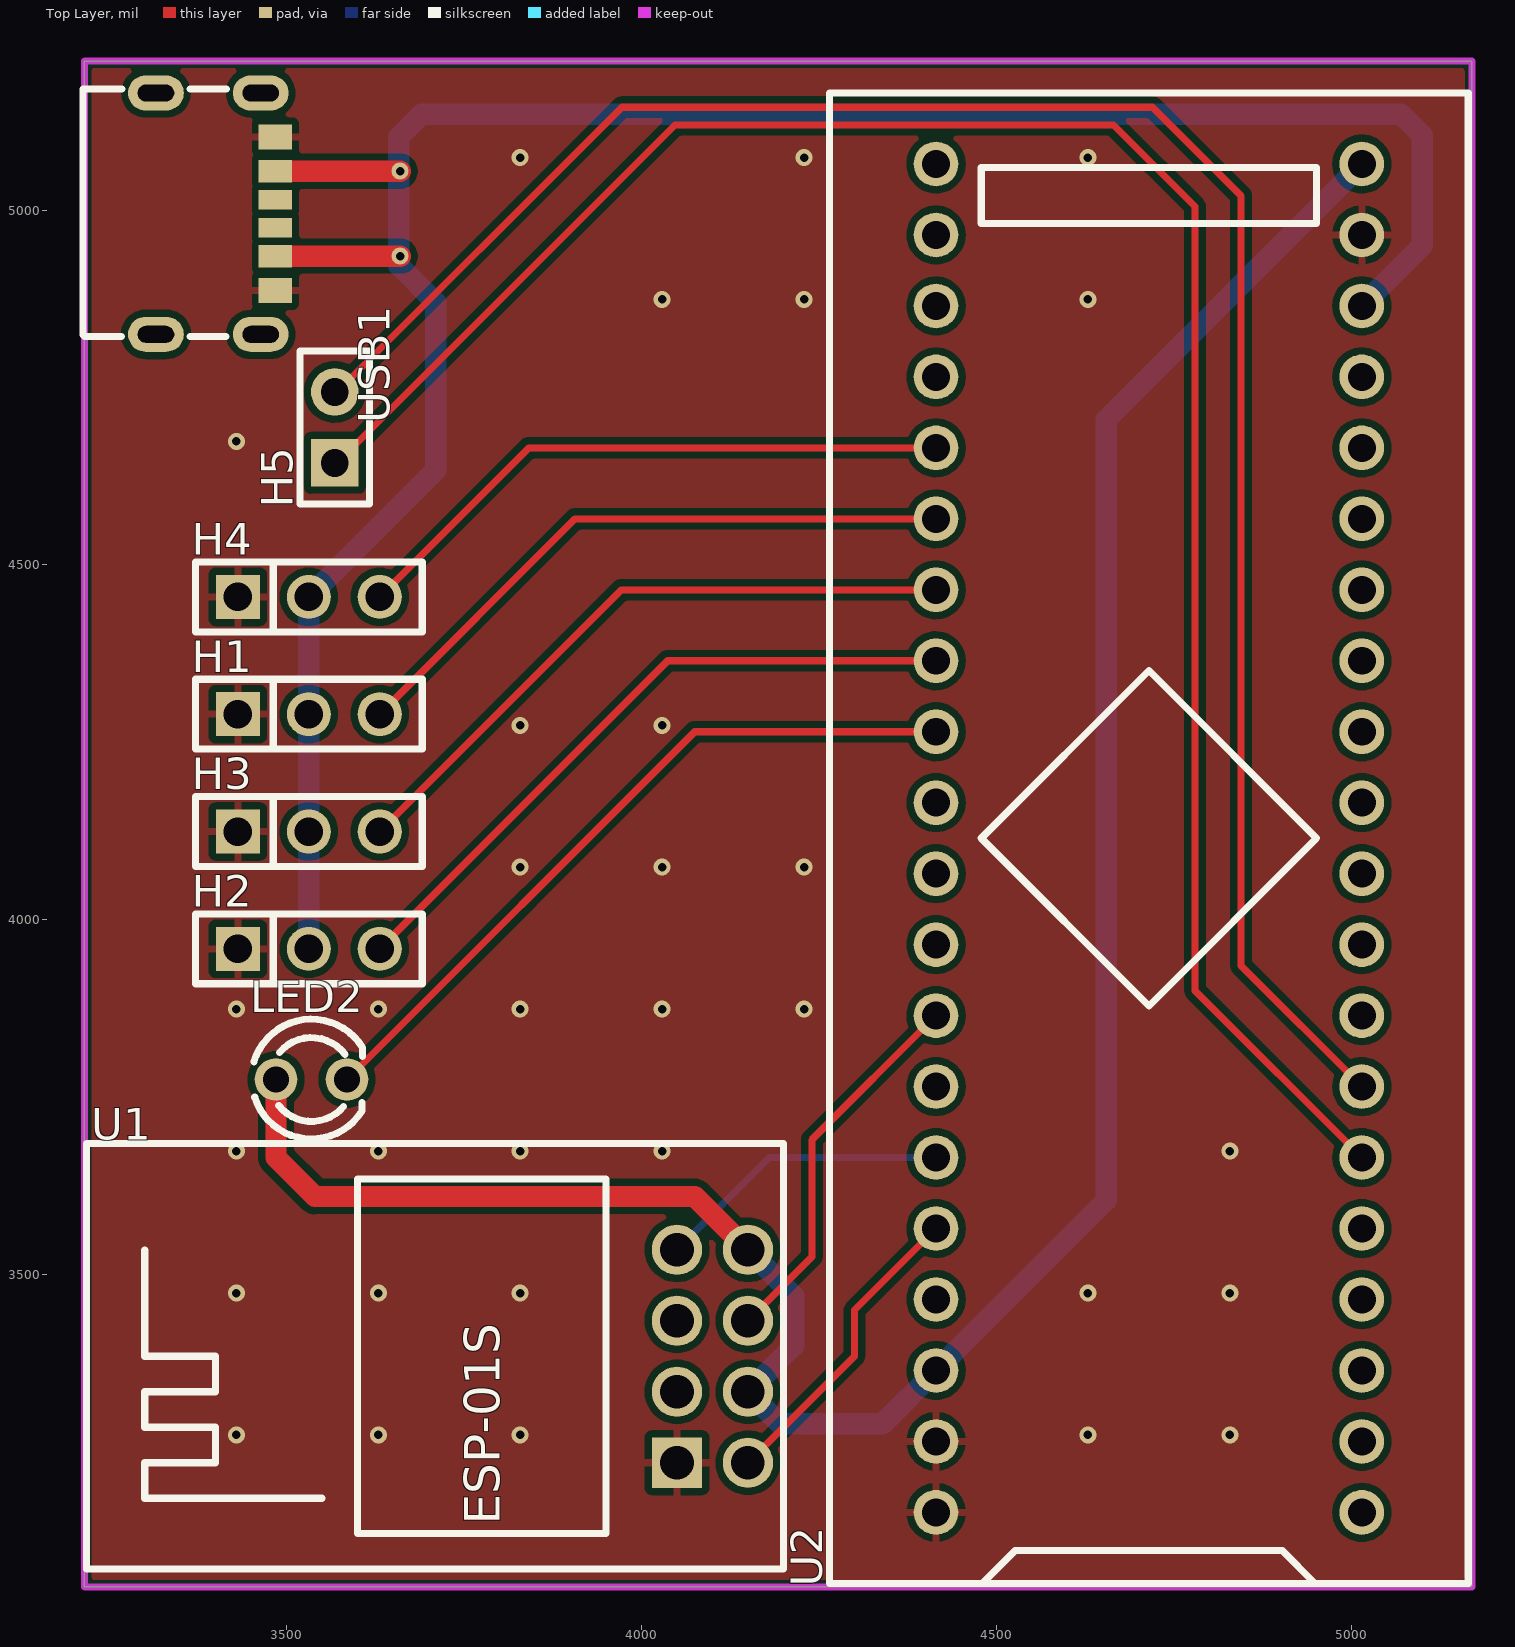
[diagram p0: Top Layer view]
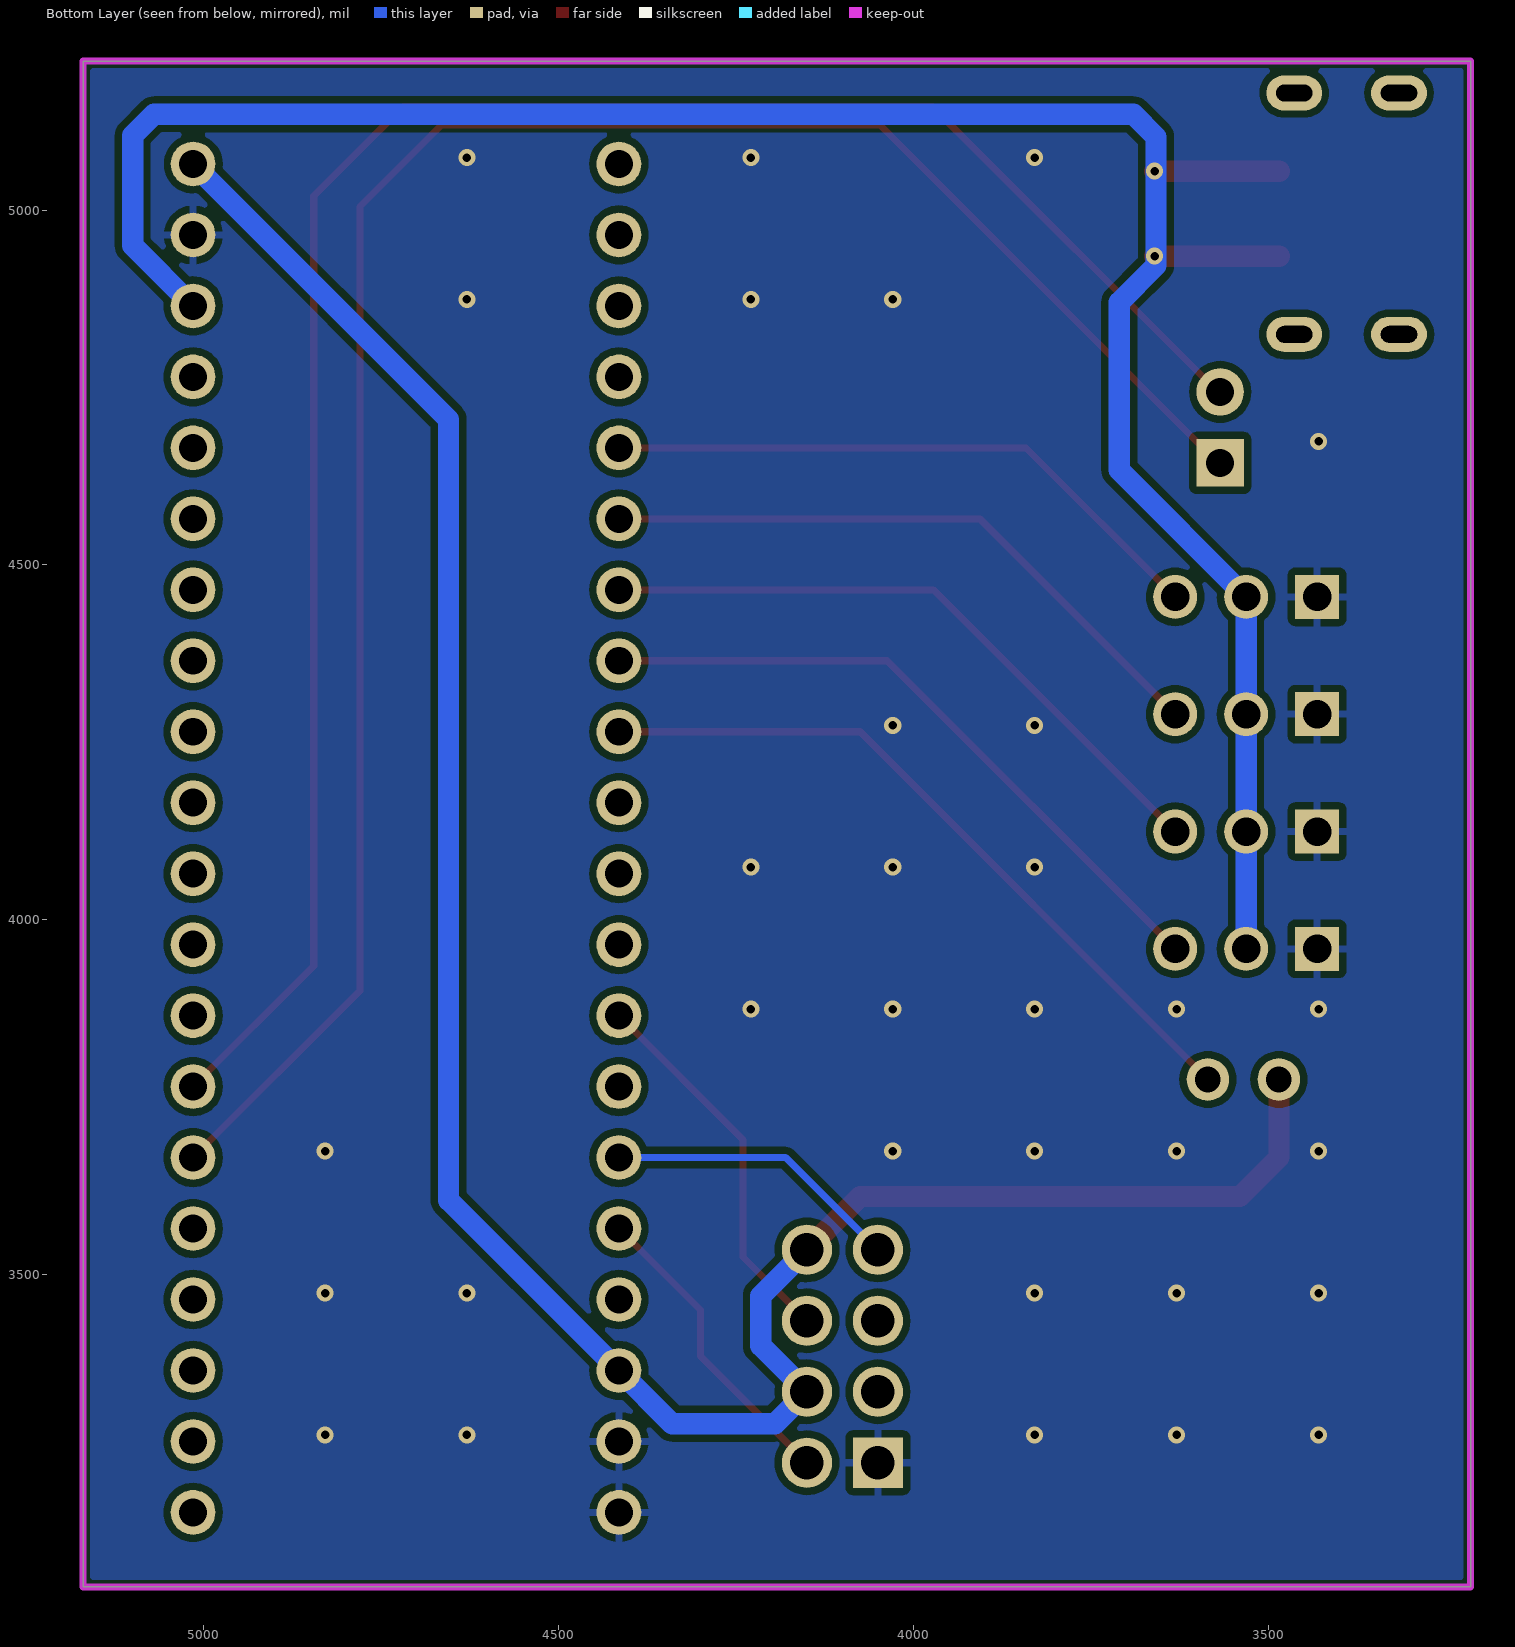
[diagram p1: Bottom Layer view, seen from below]
# Altium PCB MISC51955.pcbdoc
Units mil, origin at the board's own origin, x right, y up, seen from the top; angles counter-clockwise.
Board outline 1955 x 2150 mil, 2 copper layers (Top Layer, Bottom Layer), stack 62.206 mil thick; 9 components, 13 nets, 74 pads, 34 vias.

## Layer stack, top to bottom
Top Solder Mask Layer: solder mask 0.394, Dk 3.3
Top Layer: signal copper 1.379
Dielectric1: surface 59.449, FR4, Dk 4.5
Bottom Layer: signal copper 1.378
Bottom Solder Mask Layer: solder mask 0.394, Dk 3.3

## Board outline
3215,5210 3215,3060 5170,3060 5170,5210

## Design rules (kind name [scope] priority, off if disabled: settings)
BoardOutlineClearance copperThickness2oz_1 [All] p2 off: genericclearance=7.99 ignorepadtopadclearanceinfootprint=FALSE except(0: Arc-SplitContinuation Track-SplitContinuation SMDPad-SplitContinuation THPad-SplitContinuation Via-SplitContinuation Fill-SplitContinuation Region-SplitContinuation Poly-SplitContinuation Text-SplitContinuation Hole-SplitContinuation; 5.98: Arc-CutoutEdge SMDPad-CutoutEdge THPad-CutoutEdge Via-CutoutEdge Fill-CutoutEdge Region-CutoutEdge Text-CutoutEdge; 6.93: Hole-OutlineEdge Hole-CutoutEdge; 10: Poly-OutlineEdge Poly-CutoutEdge; 11.81: Arc-OutlineEdge Track-OutlineEdge SMDPad-OutlineEdge THPad-OutlineEdge Via-OutlineEdge Fill-OutlineEdge Region-OutlineEdge Text-OutlineEdge Track-CutoutEdge)
BoardOutlineClearance Plane_innerPlane_1 [All] p4 off: genericclearance=4.02 ignorepadtopadclearanceinfootprint=FALSE except(0: Arc-SplitContinuation Track-SplitContinuation SMDPad-SplitContinuation THPad-SplitContinuation Via-SplitContinuation Fill-SplitContinuation Region-SplitContinuation Poly-SplitContinuation Text-SplitContinuation Hole-SplitContinuation; 6: SMDPad-CutoutEdge THPad-CutoutEdge Via-CutoutEdge Fill-CutoutEdge Region-CutoutEdge Text-CutoutEdge; 6.93: Hole-OutlineEdge Hole-CutoutEdge; 10: Poly-OutlineEdge Poly-CutoutEdge; 11.8: Arc-OutlineEdge Track-OutlineEdge SMDPad-OutlineEdge THPad-OutlineEdge Via-OutlineEdge Fill-OutlineEdge Region-OutlineEdge Text-OutlineEdge; 11.81: Arc-CutoutEdge Track-CutoutEdge)
BoardOutlineClearance Copper_copperRegion_1 [All] p6 off: genericclearance=4.02 ignorepadtopadclearanceinfootprint=FALSE except(0: Arc-SplitContinuation Track-SplitContinuation SMDPad-SplitContinuation THPad-SplitContinuation Via-SplitContinuation Fill-SplitContinuation Region-SplitContinuation Poly-SplitContinuation Text-SplitContinuation Hole-SplitContinuation; 6: SMDPad-CutoutEdge THPad-CutoutEdge Via-CutoutEdge Fill-CutoutEdge Region-CutoutEdge Text-CutoutEdge; 6.93: Hole-OutlineEdge Hole-CutoutEdge; 10: Poly-OutlineEdge Poly-CutoutEdge; 11.8: Arc-OutlineEdge Track-OutlineEdge SMDPad-OutlineEdge THPad-OutlineEdge Via-OutlineEdge Fill-OutlineEdge Region-OutlineEdge Text-OutlineEdge; 11.81: Arc-CutoutEdge Track-CutoutEdge)
BoardOutlineClearance copperThickness1oz_1 [All] p8: genericclearance=4.02 ignorepadtopadclearanceinfootprint=FALSE except(0: Arc-SplitContinuation Track-SplitContinuation SMDPad-SplitContinuation THPad-SplitContinuation Via-SplitContinuation Fill-SplitContinuation Region-SplitContinuation Poly-SplitContinuation Text-SplitContinuation Hole-SplitContinuation; 6: SMDPad-CutoutEdge THPad-CutoutEdge Via-CutoutEdge Fill-CutoutEdge Region-CutoutEdge Text-CutoutEdge; 6.93: Hole-OutlineEdge Hole-CutoutEdge; 10: Poly-OutlineEdge Poly-CutoutEdge; 11.8: Arc-OutlineEdge Track-OutlineEdge SMDPad-OutlineEdge THPad-OutlineEdge Via-OutlineEdge Fill-OutlineEdge Region-OutlineEdge Text-OutlineEdge; 11.81: Arc-CutoutEdge Track-CutoutEdge)
Clearance copperThickness2oz [All] p1 off: gap=7.99 ignorepadtopadclearanceinfootprint=FALSE except(5.98: SMDPad-Track SMDPad-SMDPad THPad-Track SMDPad-THPad THPad-THPad Track-Via SMDPad-Via THPad-Via Via-Via Fill-Track Region-Track Fill-SMDPad Region-SMDPad Fill-THPad Region-THPad Fill-Via Region-Via Fill-Fill Fill-Region Region-Region Arc-Track Arc-SMDPad Arc-THPad Arc-Via Fill-Arc Region-Arc Arc-Arc Text-Track SMDPad-Text Text-THPad Text-Via Fill-Text Region-Text Arc-Text Text-Text; 6.93: Hole-Track Hole-SMDPad Hole-THPad Hole-Via Fill-Hole Region-Hole Hole-Arc Hole-Text; 10: Poly-Track Poly-SMDPad Poly-THPad Poly-Via Poly-Fill Poly-Region Poly-Poly Poly-Arc Poly-Text Poly-Hole)
Clearance Plane_innerPlane [All] p3 off: gap=4.02 ignorepadtopadclearanceinfootprint=FALSE except(5.98: SMDPad-Track SMDPad-SMDPad THPad-Track SMDPad-THPad THPad-THPad Track-Via SMDPad-Via THPad-Via Via-Via Fill-Track Region-Track Fill-SMDPad Region-SMDPad Fill-THPad Region-THPad Fill-Via Region-Via Fill-Fill Fill-Region Region-Region; 6: Arc-Track Arc-SMDPad Arc-THPad Arc-Via Fill-Arc Region-Arc Arc-Arc Text-Track SMDPad-Text Text-THPad Text-Via Fill-Text Region-Text Arc-Text Text-Text; 6.93: Hole-Track Hole-SMDPad Hole-THPad Hole-Via Fill-Hole Region-Hole Hole-Arc Hole-Text; 10: Poly-Track Poly-SMDPad Poly-THPad Poly-Via Poly-Fill Poly-Region Poly-Poly Poly-Arc Poly-Text Poly-Hole)
Clearance Copper_copperRegion [All] p5 off: gap=4.02 ignorepadtopadclearanceinfootprint=FALSE except(5.98: SMDPad-Track SMDPad-SMDPad THPad-Track SMDPad-THPad THPad-THPad Track-Via SMDPad-Via THPad-Via Via-Via Fill-Track Region-Track Fill-SMDPad Region-SMDPad Fill-THPad Region-THPad Fill-Via Region-Via Fill-Fill Fill-Region Region-Region; 6: Arc-Track Arc-SMDPad Arc-THPad Arc-Via Fill-Arc Region-Arc Arc-Arc Text-Track SMDPad-Text Text-THPad Text-Via Fill-Text Region-Text Arc-Text Text-Text; 6.93: Hole-Track Hole-SMDPad Hole-THPad Hole-Via Fill-Hole Region-Hole Hole-Arc Hole-Text; 10: Poly-Track Poly-SMDPad Poly-THPad Poly-Via Poly-Fill Poly-Region Poly-Poly Poly-Arc Poly-Text Poly-Hole)
Clearance copperThickness1oz [All] p7: gap=4.02 ignorepadtopadclearanceinfootprint=FALSE except(5.98: SMDPad-Track SMDPad-SMDPad THPad-Track SMDPad-THPad THPad-THPad Track-Via SMDPad-Via THPad-Via Via-Via Fill-Track Region-Track Fill-SMDPad Region-SMDPad Fill-THPad Region-THPad Fill-Via Region-Via Fill-Fill Fill-Region Region-Region; 6: Arc-Track Arc-SMDPad Arc-THPad Arc-Via Fill-Arc Region-Arc Arc-Arc Text-Track SMDPad-Text Text-THPad Text-Via Fill-Text Region-Text Arc-Text Text-Text; 6.93: Hole-Track Hole-SMDPad Hole-THPad Hole-Via Fill-Hole Region-Hole Hole-Arc Hole-Text; 10: Poly-Track Poly-SMDPad Poly-THPad Poly-Via Poly-Fill Poly-Region Poly-Poly Poly-Arc Poly-Text Poly-Hole)
DiffPairsRouting differentialPair [All] p1: maxlimit=6 minlimit=6 mostfreqgap=6 toplayer_minwidth=5 toplayer_prefwidth=10 toplayer_maxwidth=100 toplayer_mingap=6 toplayer_prefgap=6 toplayer_maxgap=6 bottomlayer_minwidth=5 bottomlayer_prefwidth=10 bottomlayer_maxwidth=100 bottomlayer_mingap=6 bottomlayer_prefgap=6 bottomlayer_maxgap=6 maxuncoupledlength=10
HoleToHoleClearance otherClearance [All] p1: gap=11.81 allowstackedmicrovias=TRUE
Length netLength [All] p1: minlimit=0 maxlimit=0
PasteMaskExpansion pasteMaskExpansion [All] p1: expansion=0
PlaneConnect innerPlane [All] p1: planeconnectstyle=Relief reliefexpansion=20 reliefentries=4 reliefconductorwidth=10 reliefairgap=10
PolygonConnect copperRegion [All] p1: connectstyle=Relief reliefconductorwidth=10 reliefentries=4 polygonreliefangle="90 Angle" airgapwidth=10 via.connectstyle=Relief via.reliefconductorwidth=10 via.reliefentries=4 via.polygonreliefangle="90 Angle" via.airgapwidth=10
RoutingVias viaSize [All] p1: holewidth=12.01 width=24.02 viastyle="Through Hole" minholewidth=11.81 minwidth=19.68 maxholewidth=248.03 maxwidth=393.7
SolderMaskExpansion solderMaskExpansion [IsVia] p1: expansion=-1000 istentingtop=TRUE
SolderMaskExpansion solderMaskExpansion [All] p2: expansion=2 istentingtop=FALSE
Width copperThickness2oz_2 [All] p1 off: maxlimit=100 minlimit=8 preferedwidth=10
Width copperThickness1oz_2 [All] p2: maxlimit=100 minlimit=5 preferedwidth=10

## Components (designator, comment, footprint, x,y, rotation, side; value= is the part's Value field where it differs from the comment)
H1 "" HDR-TH_3P-P2.54-V-F 3531.17,4289.71 r0 top
H2 "" HDR-TH_3P-P2.54-V-F 3531.17,3959.14 r0 top
H3 "" HDR-TH_3P-P2.54-V-F 3531.17,4124.43 r0 top
H4 "" HDR-TH_3P-P2.54-V-F 3531.17,4455 r0 top
H5 "" HDR-TH_2P-P2.54-V-F 3567.77,4693.84 r90 top
LED2 "" LED_TH-3mm 3535,3775 r0 top
U1 "ESP-01S" WIFIM-TH_ESP-01S 4100,3385 r90 top
U2 "STM32F103C8T6最小系统开发板" CONN-TH_L53.3-W22.9_STM32F103C8T6-CARD 4715,4115 r90 top
USB1 "" "USB_ TYPE-C-6P" 3400,5000 r270 top

## Footprints (in the part's own frame and the unit in brackets; to place one, negate y for a bottom-side part, rotate by r counter-clockwise, add the part's x,y. Pads: shape width x height; smd on the part's side, far side on the other; paste and mask are expansions set on the pad)
CONN-TH_L53.3-W22.9_STM32F103C8T6-CARD [mm]
  round 1.6 hole 1: 1(-24.13,-7.62) 2(-21.59,-7.62) 3(-19.05,-7.62) 4(-16.51,-7.62) 5(-13.97,-7.62) 6(-11.43,-7.62) 7(-8.89,-7.62) 8(-6.35,-7.62) 9(-3.81,-7.62) 10(-1.27,-7.62) 11(1.27,-7.62) 12(3.81,-7.62) 13(6.35,-7.62) 14(8.89,-7.62) 15(11.43,-7.62) 16(13.97,-7.62) 17(16.51,-7.62) 18(19.05,-7.62) 19(21.59,-7.62) 20(24.13,-7.62) 21(24.13,7.62) 22(21.59,7.62) 23(19.05,7.62) 24(16.51,7.62) 25(13.97,7.62) 26(11.43,7.62) 27(8.89,7.62) 28(6.35,7.62) 29(3.81,7.62) 30(1.27,7.62) 31(-1.27,7.62) 32(-3.81,7.62) 33(-6.35,7.62) 34(-8.89,7.62) 35(-11.43,7.62) 36(-13.97,7.62) 37(-16.51,7.62) 38(-19.05,7.62) 39(-21.59,7.62) 40(-24.13,7.62)
  silkscreen extent -26.67,-11.43 26.67,11.43
HDR-TH_2P-P2.54-V-F [mm]
  rect 1.7x1.7 hole 1: 1(-1.27,0)
  round 1.7 hole 1: 2(1.27,0)
  silkscreen extent -2.74,-1.25 2.74,1.25
HDR-TH_3P-P2.54-V-F [mil]
  rect 62x62 hole 40.16: 1(-100,0)
  round 62 hole 40.16: 2(0,0) 3(100,0)
  silkscreen extent -160,-49 160,49
LED_TH-3mm [mil]
  round 60 hole 36 paste+0 mask+2: 1(-50,0) 2(50,0)
  silkscreen extent -81,-84 72,85
"USB_ TYPE-C-6P" [mm]
  oval 1.25x2 hole 0.6 slot 1.3 at 90 deg paste+0 mask+0.05: 7(-4.193,1.611) 8(4.447,1.611) 9(-4.193,-2.139) 10(4.447,-2.139)
  rect 0.7x1.2 smd paste-100 mask+0.05: A5(-0.373,2.139) B5(0.627,2.139)
  rect 0.8x1.2 smd paste-100 mask+0.05: A9(1.647,2.139) B9(-1.393,2.139)
  rect 0.9x1.2 smd paste-100 mask+0.05: A12(2.877,2.139) B12(-2.623,2.139)
  silkscreen extent -4.34,-4.75 4.52,0.39
WIFIM-TH_ESP-01S [mm]
  rect 1.8x1.8 hole 1.2: 1(-3.81,1.27)
  round 1.8 hole 1.2: 2(-1.27,1.27) 3(1.27,1.27) 4(3.81,1.27) 5(3.81,-1.27) 6(1.27,-1.27) 7(-1.27,-1.27) 8(-3.81,-1.27)
  silkscreen extent -7.62,-2.54 7.62,22.4

## Via types
v1: diameter 24.02, hole 12, Top Layer to Bottom Layer, 34 vias

## Nets (pads, with @x,y where several pads share a name; then routed paths per layer and width w, separated by ;. In a path a pad name is that pad's centre, name@x,y a point inside that pad or via, vN(x,y) a via of type N, cw(c..) or ccw(c..) an arc to the next point about the centre after c; other vN are vias at no path point)
+5V: H1.2 H2.2 H3.2 H4.2 U2.18 USB1.A9 USB1.B9 | length 3333.8
  Top Layer w30: USB1.A9 v1(3660,4935.16) ; USB1.B9 v1(3660,5054.84)
  Bottom Layer w30: H2.2 H3.2 H1.2 H4.2 3710,4633.83 3710,4870 3658.1,4921.9 3658.1,5103.1 3690,5135 5070,5135 5100,5105 5100,4950 U2.18
GND: H1.1 H2.1 H3.1 H4.1 U1.1 U2.19 U2.39 U2.40 USB1.A12 USB1.B12
  other v1: 3429.1,3274.1 3629.1,3274.1 3829.1,3274.1 4629.1,3274.1 4829.1,3274.1 3429.1,3474.1 3629.1,3474.1 3829.1,3474.1 4629.1,3474.1 4829.1,3474.1 3429.1,3674.1 3629.1,3674.1 3829.1,3674.1 4029.1,3674.1 4829.1,3674.1 3429.1,3874.1 3629.1,3874.1 3829.1,3874.1 4029.1,3874.1 4229.1,3874.1 3829.1,4074.1 4029.1,4074.1 4229.1,4074.1 3829.1,4274.1 4029.1,4274.1 3429.1,4674.1 4029.1,4874.1 4229.1,4874.1 4629.1,4874.1 3829.1,5074.1 4229.1,5074.1 4629.1,5074.1
PA0: H4.3 U2.25 | length 870.8
  Top Layer w10: H4.3 3841.17,4665 U2.25
PA1: H1.3 U2.26 | length 897.9
  Top Layer w10: H1.3 3906.46,4565 U2.26
PA2: H3.3 U2.27 | length 924.9
  Top Layer w10: H3.3 3971.74,4465 U2.27
PA3: H2.3 U2.28 | length 951.9
  Top Layer w10: H2.3 4037.03,4365 U2.28
PA4: LED2.2 U2.29 | length 1033
  Top Layer w10: LED2.2 4075,4265 U2.29
PA9: H5.1 U2.6 | length 2894.3
  Top Layer w10: H5.1@3568.88,4641.58 4047.3,5120 4665,5120 4780,5005 4780,3900 U2.6
PA10: H5.2 U2.7 | length 2820.4
  Top Layer w10: H5.2@3568.88,4741.58 3972.3,5145 4720,5145 4845,5020 4845,3935 U2.7
PB0: U1.6 U2.33 | length 539.8
  Top Layer w10: U1.6 4240,3525 4240,3690 U2.33
PB10: U1.4 U2.35 | length 418.8
  Bottom Layer w10: U1.4 4180,3665 U2.35
PB11: U1.8 U2.36 | length 439.8
  Top Layer w10: U1.8 4300,3385 4300,3450 U2.36
VCC: LED2.1 U1.5 U1.7 U2.20 U2.38 | length 3345.9
  Top Layer w30: LED2.1 3485,3665 3540,3610 4075,3610 U1.5
  Bottom Layer w30: U1.5 4215,3470 4215,3400 U1.7 4195,3290 4340,3290 U2.38 4655,3605 4655,4705 U2.20
pads on no net: U1.2 U1.3 U2.1 U2.2 U2.3 U2.4 U2.5 U2.8 U2.9 U2.10 U2.11 U2.12 U2.13 U2.14 U2.15 U2.16 U2.17 U2.21 U2.22 U2.23 U2.24 U2.30 U2.31 U2.32 U2.34 U2.37 USB1.7 USB1.8 USB1.9 USB1.10 USB1.A5 USB1.B5

## Polygon pours and split planes (outlines as drawn)
GND on Bottom Layer (solid, remove dead copper, pour order 2): 3000,5320 3000,3030 5405,3030 5405,5320
GND on Top Layer (solid, remove dead copper, pour order 0): 3055,5305 3055,3000 5470,3000 5470,5305

## Keep-outs
Board Outline Layer:
  the board outline again, w10